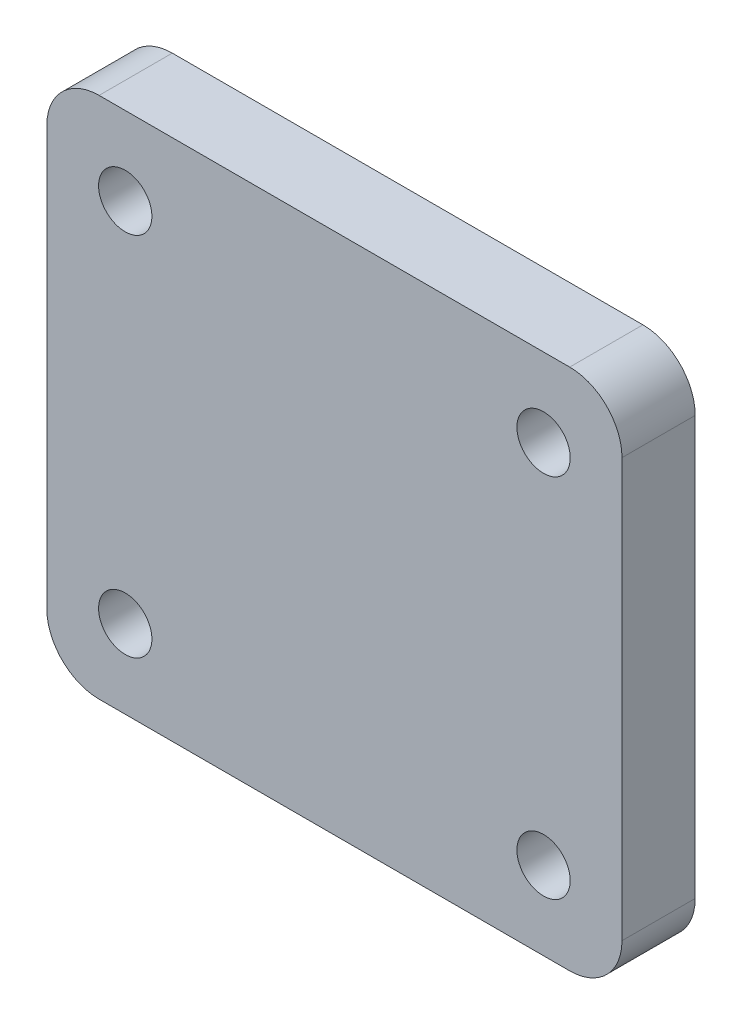
from build123d import *

# Parameters (mm, degrees)
EXTRUDE_1_DEPTH         = 14
HOLE_WIZARD_M12_1_D     = 10.2
HOLE_WIZARD_M12_1_DEPTH = 29.25
HOLE_WIZARD_M12_1_TIP   = 3.064389157


with BuildPart() as part:
    # 草图1 → 凸台-拉伸1 (new body)
    with BuildSketch(Plane.XY):
        with BuildLine():
            Line((10, 0), (100, 0))
            ThreePointArc((100, 0), (107.071067812, 2.928932188), (110, 10))
            Line((110, 10), (110, 90))
            ThreePointArc((110, 90), (107.071067812, 97.071067812), (100, 100))
            Line((100, 100), (10, 100))
            ThreePointArc((10, 100), (2.928932188, 97.071067812), (0, 90))
            Line((0, 90), (0, 10))
            ThreePointArc((0, 10), (2.928932188, 2.928932188), (10, 0))
        make_face()
    extrude(amount=EXTRUDE_1_DEPTH)

    # M12 螺纹孔1
    with Locations(Plane(origin=(15, 85, 14), x_dir=(1, 0, 0), z_dir=(0, 0, 1))):
        with Locations((0, 0), (80, 0), (80, -70), (0, -70)):
            Hole(HOLE_WIZARD_M12_1_D / 2, depth=HOLE_WIZARD_M12_1_DEPTH)
            with Locations((0, 0, -(HOLE_WIZARD_M12_1_DEPTH + HOLE_WIZARD_M12_1_TIP / 2))):  # 118° drill point
                Cone(0, HOLE_WIZARD_M12_1_D / 2, HOLE_WIZARD_M12_1_TIP, mode=Mode.SUBTRACT)


solid = part.part
